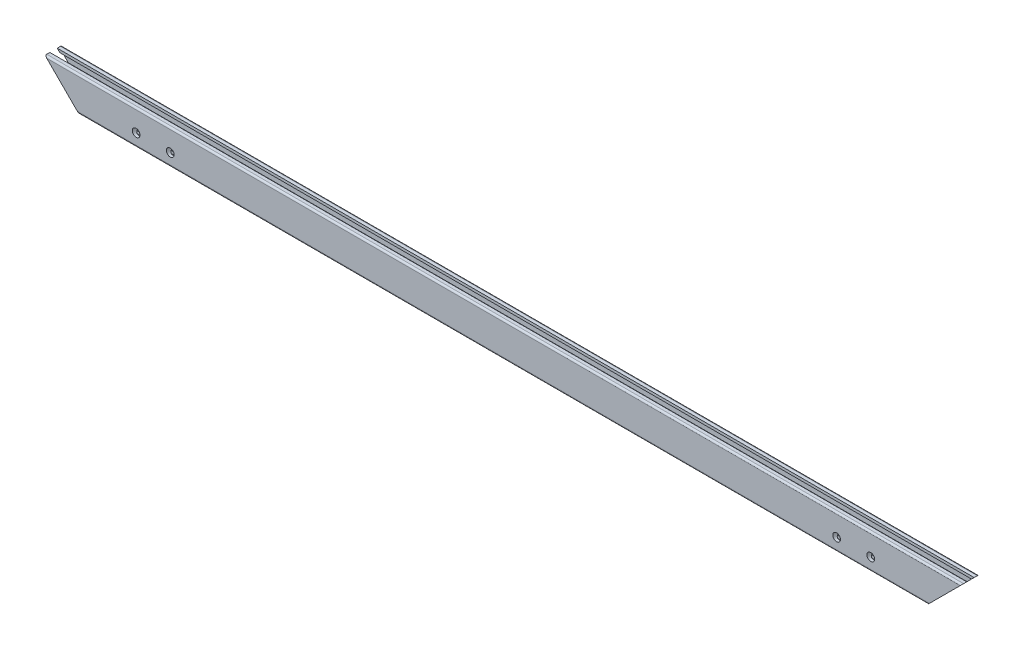
from build123d import *

# Parameters (mm, degrees)
SKETCH11_R          = 2.5
MEMBER_1_DEPTH      = 805
CUT_EXTRUDE_1_DEPTH = 404.058618566
HOLE_WIZARD_M8_1_D  = 6.8


with BuildPart() as part:
    # Sketch11 → Member 1 (new body)
    with BuildSketch(Plane(origin=(-402.5, 0, 0), x_dir=(0, 0, -1), z_dir=(1, 0, 0))):
        with BuildLine():
            Line((-6, -15), (-3.25, -15))
            Line((-3.25, -15), (-3.25, -12.7))
            Line((-3.25, -12.7), (-5, -12.7))
            Line((-5, -12.7), (-5, -7))
            ThreePointArc((-5, -7), (0, -4.31662479), (5, -7))
            Line((5, -7), (5, -12.7))
            Line((5, -12.7), (3.25, -12.7))
            Line((3.25, -12.7), (3.25, -15))
            Line((3.25, -15), (6, -15))
            ThreePointArc((6, -15), (7.060660172, -14.560660172), (7.5, -13.5))
            Line((7.5, -13.5), (7.5, 13.5))
            ThreePointArc((7.5, 13.5), (7.060660172, 14.560660172), (6, 15))
            Line((6, 15), (3.25, 15))
            Line((3.25, 15), (3.25, 12.7))
            Line((3.25, 12.7), (5, 12.7))
            Line((5, 12.7), (5, 7))
            ThreePointArc((5, 7), (0, 4.31662479), (-5, 7))
            Line((-5, 7), (-5, 12.7))
            Line((-5, 12.7), (-3.25, 12.7))
            Line((-3.25, 12.7), (-3.25, 15))
            Line((-3.25, 15), (-6, 15))
            ThreePointArc((-6, 15), (-7.060660172, 14.560660172), (-7.5, 13.5))
            Line((-7.5, 13.5), (-7.5, -13.5))
            ThreePointArc((-7.5, -13.5), (-7.060660172, -14.560660172), (-6, -15))
        make_face()
        Circle(SKETCH11_R, mode=Mode.SUBTRACT)
    extrude(amount=MEMBER_1_DEPTH)

    # 草图4 → 切除-拉伸1 (cut, through all)
    with BuildSketch(Plane.XY.offset(7.5)):
        Polygon((-402.5, 15), (-372.5, -15), (-402.5, -15), align=None)
        Polygon((402.5, -15), (402.5, 15), (372.5, -15), align=None)
    extrude(amount=-CUT_EXTRUDE_1_DEPTH, mode=Mode.SUBTRACT)

    # M8 螺纹孔1 (through all)
    with Locations(Plane.XY.offset(7.5)):
        with Locations((-322.5, -4), (-292.5, -4), (292.5, -4), (322.5, -4)):
            Hole(HOLE_WIZARD_M8_1_D / 2)


solid = part.part
